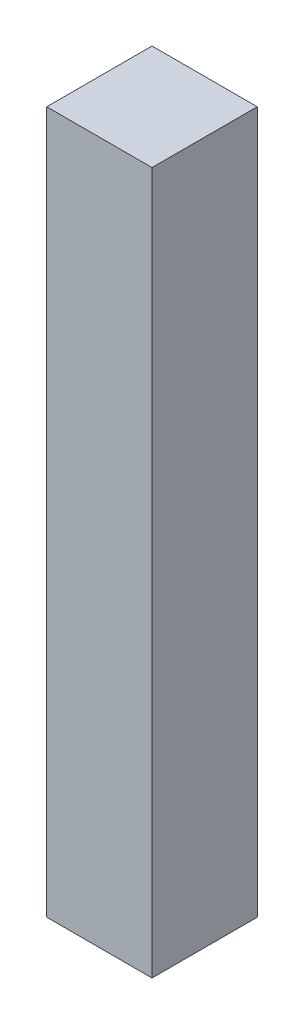
from build123d import *

# Parameters (mm, degrees)
SKETCH1_W           = 3
SKETCH1_H           = 3
BOSS_EXTRUDE1_DEPTH = 20


with BuildPart() as part:
    # Sketch1 → Boss-Extrude1 (new body)
    with BuildSketch(Plane(origin=(0, 0, 0), x_dir=(1, 0, 0), z_dir=(0, 1, 0))):
        Rectangle(SKETCH1_W, SKETCH1_H)
    extrude(amount=BOSS_EXTRUDE1_DEPTH)


solid = part.part
